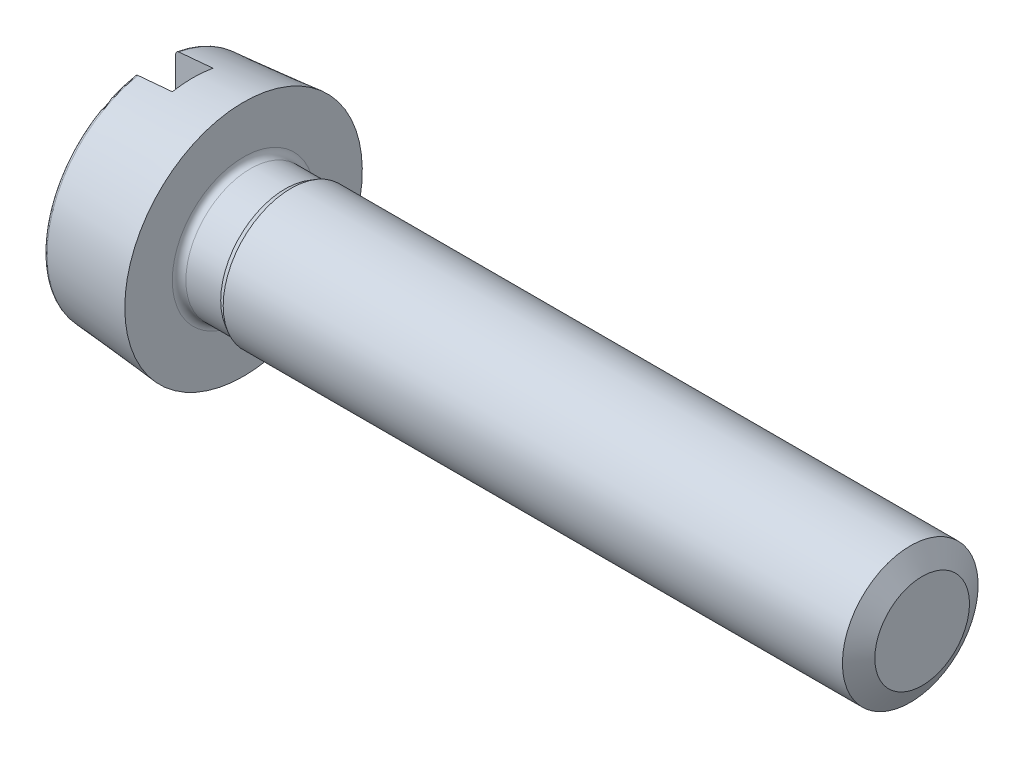
SolidWorks part; units mm, degrees
revolve "Base-Revolve" add sketch "Sketch1" angle 360 about L0
sketch "Sketch1" plane through (0, 0, 0) normal (0, 0, 1) x (1, 0, 0)
  line L0 (0, 0) -> (22.6, 0) construction
  line L1 (0, 0) -> (0, 3.1809)
  line L2 (2.6, 3.5) -> (0.0913, 3.2805)
  line L3 (2.6, 3.5) -> (2.6, 2.1)
  line L4 (2.8, 1.9) -> (3.8268, 1.9)
  line L5 (3.8268, 1.9) -> (4, 2)
  line L6 (4, 2) -> (22.6, 2)
  line L7 (22.6, 2) -> (22.6, 0)
  line L8 (0, 0) -> (22.6, 0)
  arc A0 (2.8, 1.9) -> (2.6, 2.1) centre (2.8, 2.1) cw
  arc A1 (0, 3.1809) -> (0.0913, 3.2805) centre (0.1, 3.1809) cw
cosmetic thread "Cosmetic Thread1" parameters "D1"=3.3866, "D2"=1.2
ref_plane "Front Plane" through (0, 0, 0) normal (0, 0, 1) x (1, 0, 0)
ref_plane "Top Plane" through (0, 0, 0) normal (0, 1, 0) x (1, 0, 0)
ref_plane "Right Plane" through (0, 0, 0) normal (1, 0, 0) x (0, 0, -1)
sketch "Dimension Sketch" plane through (0, 0, 0) normal (0, 0, 1) x (1, 0, 0)
  line L0 (0, 0) -> (22.6, 0)
  point P3 (1.1, 0)
  point P4 (1.4, 0)
  point P5 (4, 0)
  point P6 (7, 0)
  point P7 (1.2, 0)
  point P8 (3.1989, 0)
  point P9 (3.656, 0)
  point P10 (4.0948, 0)
  point P11 (21.9, 0)
  point P12 (22.4, 0)
  point P13 (2.6, 0)
sketch "Sketch2" plane through (0, 0, 0) normal (-1, 0, 0) x (0, 0, 1)
  line L0 (0, 0) -> (0, -1.8809) construction
  line L3 (0.6, 3.4482) -> (0.6, -3.4482)
  line L5 (-0.6, 3.4482) -> (-0.6, -3.4482)
  circle A1 centre (0, 0) radius 3.5 construction
  arc A2 (0.6, 3.4482) -> (-0.6, 3.4482) centre (0, 0) ccw
  arc A3 (-0.6, -3.4482) -> (0.6, -3.4482) centre (0, 0) ccw
extrude "Cut-Extrude1" cut sketch "Sketch2" against normal blind 1.1
sketch "Sketch3" plane through (0, 0, 0) normal (0, 1, 0) x (1, 0, 0)
  line L0 (22.25, 2) -> (22.95, 2)
  line L2 (22.95, 2) -> (22.6, 1.3938)
  line L3 (22.6, 1.3938) -> (22.25, 2)
  line L4 (22.6, -1.6037) -> (22.6, 3.368) construction
  line L10 (22.6, -2) -> (22.6, 2) construction
  line L11 (0, 0) -> (7.2232, 0) construction
revolve "Cut-Revolve1" cut sketch "Sketch3" angle 360 about L11
pattern_linear "LPattern1" [suppressed] count 28 along (1, 0, 0)
equation "\"l@Sketch1\" = \"l@Dimension Sketch\" "
equation "\"a@Sketch1\" = \"a@Dimension Sketch\" "
equation "\"r@Sketch1\" = \"r@Dimension Sketch\" "
equation "\"d@Sketch1\" = \"d@Dimension Sketch\" "
equation "\"k@Sketch1\" = \"k@Dimension Sketch\" "
equation "\"dk@Sketch1\" = \"dk@Dimension Sketch\" "
equation "\"n@Sketch2\" = \"n@Dimension Sketch\" "
equation "\"t@Cut-Extrude1\" = \"t@Dimension Sketch\" "
equation "\"D2@Sketch3\" = \"p@Dimension Sketch\" * 0.866"
equation "\"D3@Sketch3\" = \"d@Sketch1\" / 2"
equation "\"D1@Sketch1\" = \"d@Sketch1\" - \"r@Sketch1\""
equation "\"D1@LPattern1\" =  ( \"l@Sketch1\" - \"a@Sketch1\" )  / \"p@LPattern1\" + 1"
